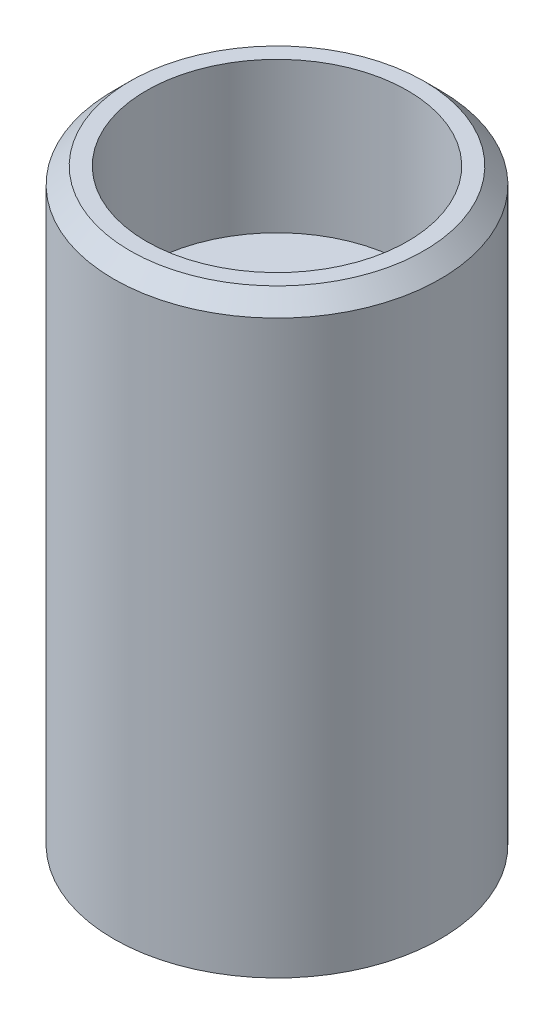
from build123d import *

# Parameters (mm, degrees)
SKETCH1_R                                          = 5
BOSS_EXTRUDE1_DEPTH                                = 18
HOLE_WIZARD_SOCKET_HEAD_CAP_SCREW_TYPE_D           = 4.5
HOLE_WIZARD_SOCKET_HEAD_CAP_SCREW_TYPE_CBORE_D     = 8
HOLE_WIZARD_SOCKET_HEAD_CAP_SCREW_TYPE_CBORE_DEPTH = 4.6
CHAMFER1_SIZE                                      = 0.5


with BuildPart() as part:
    # Sketch1 → Boss-Extrude1 (new body)
    with BuildSketch(Plane(origin=(0, 0, 0), x_dir=(1, 0, 0), z_dir=(0, 1, 0))):
        with Locations(Location((0, 0, 0), (0, 0, 270))):
            Circle(SKETCH1_R)
    extrude(amount=BOSS_EXTRUDE1_DEPTH)

    # Hole wizard: socket head cap screw, type 1 (through all)
    with Locations(Plane(origin=(0, 18, 0), x_dir=(1, 0, 0), z_dir=(0, 1, 0))):
        with Locations((0, 0)):
            CounterBoreHole(HOLE_WIZARD_SOCKET_HEAD_CAP_SCREW_TYPE_D / 2, HOLE_WIZARD_SOCKET_HEAD_CAP_SCREW_TYPE_CBORE_D / 2, HOLE_WIZARD_SOCKET_HEAD_CAP_SCREW_TYPE_CBORE_DEPTH)

    # Chamfer1
    chamfer1_edges = [part.edges().sort_by_distance(p)[0] for p in [
        (0, 18, -5),
    ]]
    chamfer(chamfer1_edges, length=CHAMFER1_SIZE)


solid = part.part
